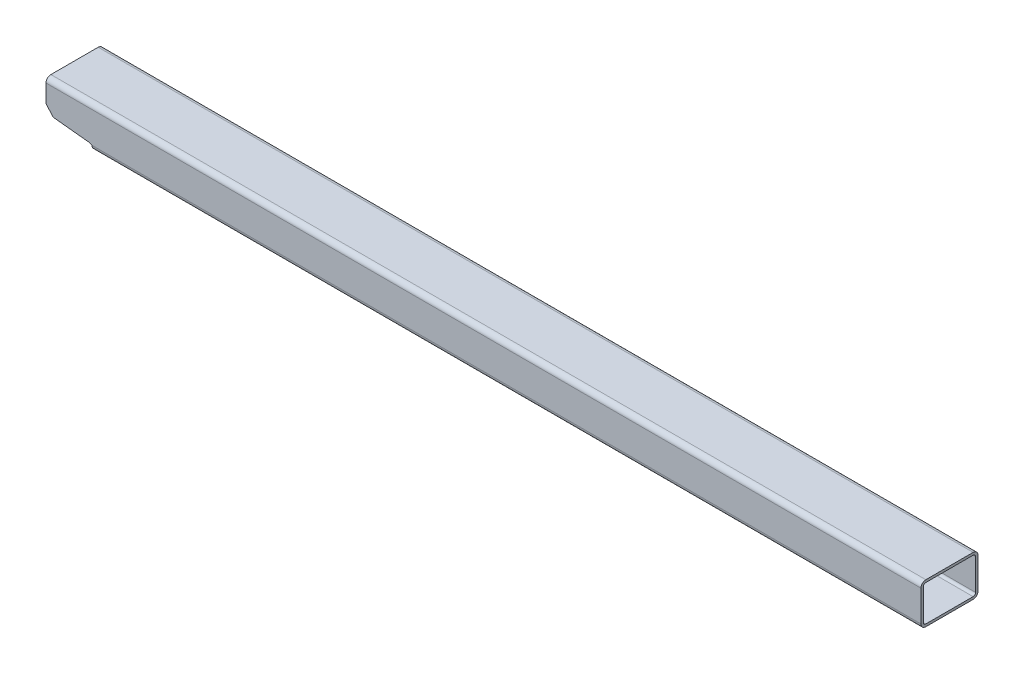
from build123d import *

# Parameters (mm, degrees)
GB_6728_1986_070_X_50_X_3_1_DEPTH = 1139.5
CUT_EXTRUDE_1_DEPTH               = 575.578160479
CUT_EXTRUDE_1_DEPTH_BACK          = 575.578160479
SKETCH_5_W                        = 71
SKETCH_5_H                        = 60
CUT_EXTRUDE_4_DEPTH               = 575.578160479


with BuildPart() as part:
    # Sketch1 → Gb／6728-1986矩形空心型钢 070 X 50 X 3(1) (new body)
    with BuildSketch(Plane.YZ.offset(-569.75)):
        with BuildLine():
            Line((-19, -35), (19, -35))
            ThreePointArc((19, -35), (23.242640687, -33.242640687), (25, -29))
            Line((25, -29), (25, 29))
            ThreePointArc((25, 29), (23.242640687, 33.242640687), (19, 35))
            Line((19, 35), (-19, 35))
            ThreePointArc((-19, 35), (-23.242640687, 33.242640687), (-25, 29))
            Line((-25, 29), (-25, -29))
            ThreePointArc((-25, -29), (-23.242640687, -33.242640687), (-19, -35))
        make_face()
        with BuildLine():
            Line((-19, -32), (19, -32))
            ThreePointArc((19, -32), (21.121320344, -31.121320344), (22, -29))
            Line((22, -29), (22, 29))
            ThreePointArc((22, 29), (21.121320344, 31.121320344), (19, 32))
            Line((19, 32), (-19, 32))
            ThreePointArc((-19, 32), (-21.121320344, 31.121320344), (-22, 29))
            Line((-22, 29), (-22, -29))
            ThreePointArc((-22, -29), (-21.121320344, -31.121320344), (-19, -32))
        make_face(mode=Mode.SUBTRACT)
    extrude(amount=GB_6728_1986_070_X_50_X_3_1_DEPTH)

    # 草图2 → 切除-拉伸1 (cut, two sides: drawn at the far end of the back side and taken through both)
    with BuildSketch(Plane(origin=(0, 0, -35), x_dir=(-1, 0, 0), z_dir=(0, 0, -1)).offset(-CUT_EXTRUDE_1_DEPTH_BACK)):
        Polygon((513.25, -25), (513.25, -19), (517.727357684, -17.498605391), (560.795284633, -12.971983864), (569.75, -3.026764911), (574.75, -3.026764911), (574.75, -30), (513.25, -30), align=None)
    extrude(amount=CUT_EXTRUDE_1_DEPTH + CUT_EXTRUDE_1_DEPTH_BACK, mode=Mode.SUBTRACT)

    # 草图5 → 切除-拉伸4 (cut, through all)
    with BuildSketch(Plane.XY.offset(35)):
        with Locations((539.25, 0)):
            Rectangle(SKETCH_5_W, SKETCH_5_H)
    extrude(amount=-CUT_EXTRUDE_4_DEPTH, mode=Mode.SUBTRACT)


solid = part.part
